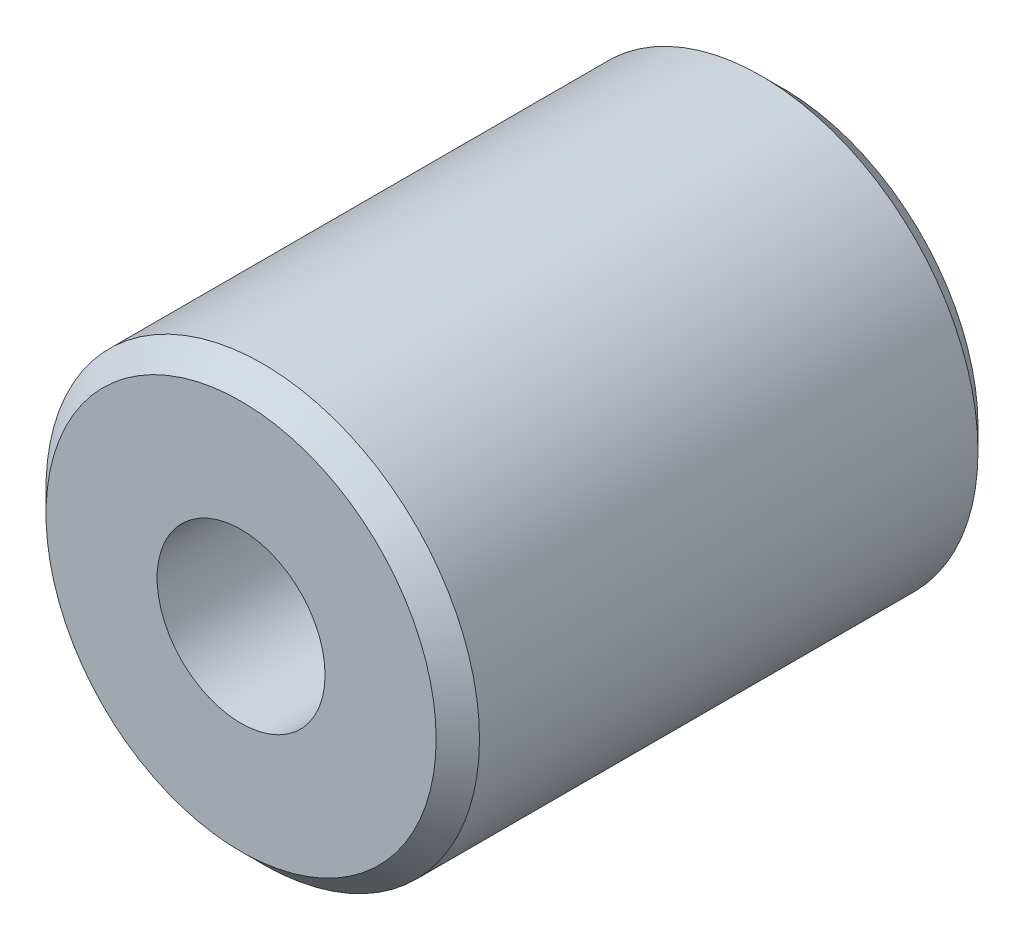
SolidWorks part; units mm, degrees
ref_plane "Front Plane" through (0, 0, 0) normal (0, 0, 1) x (1, 0, 0)
ref_plane "Top Plane" through (0, 0, 0) normal (0, 1, 0) x (1, 0, 0)
ref_plane "Right Plane" through (0, 0, 0) normal (1, 0, 0) x (0, 0, -1)
sketch "Sketch1" plane through (0, 0, 0) normal (0, 0, 1) x (1, 0, 0)
  circle A0 centre (0, 0) radius 20
  dimension "D1" = 40
extrude "Boss-Extrude1" add sketch "Sketch1" along normal mid plane 50
chamfer "Chamfer1" distance 2 angle 45 2 edges at (20, 0, -25) (20, 0, 25)
hole_wizard "M18 Tapped Hole1" positions "Sketch2" profile "Sketch3" tap size "M18" standard "GB" end condition through all
sketch "Sketch2" plane through (0, 0, 25) normal (0, 0, 1) x (1, 0, 0)
  point P0 (0, 0)
sketch "Sketch3" plane through (0, 0, 25) normal (1, 0, 0) x (0, -1, 0)
  line L0 (0, 0) -> (0, 50)
  line L1 (0, 50) -> (7.75, 50)
  line L2 (7.75, 50) -> (7.75, 0)
  line L5 (7.75, 0) -> (0, 0)
  line L11 (0, -6.35) -> (0, 107.95) construction
  dimension "通孔螺纹孔钻头直径" = 15.5
  dimension "通孔螺纹孔钻头深度" = 50
cosmetic thread "Cosmetic Thread1" parameters "D2"=18
